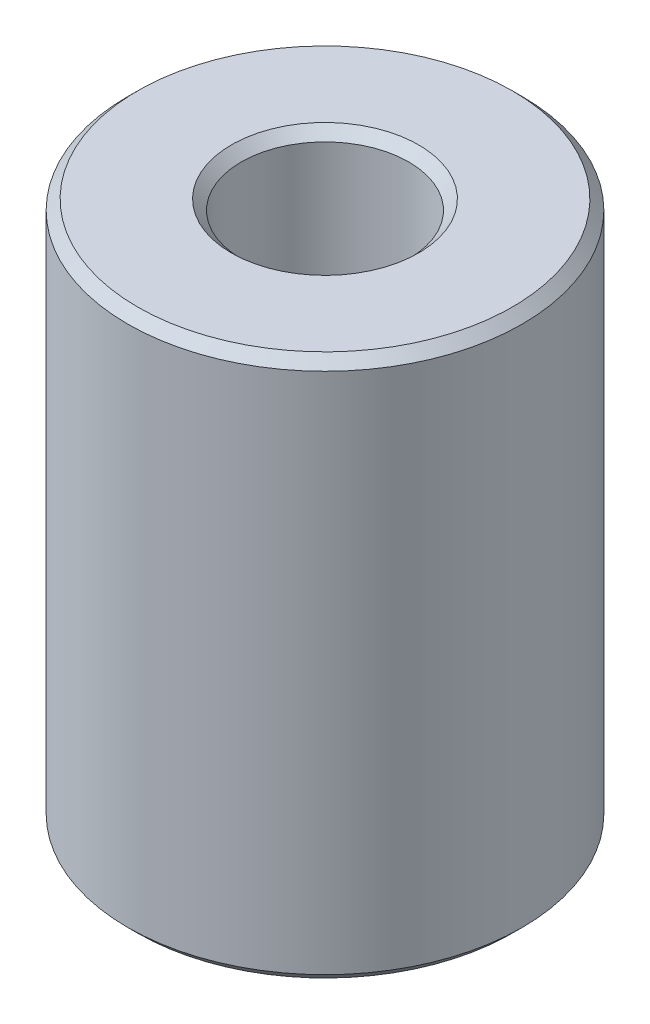
SolidWorks part; units mm, degrees
ref_plane "前视基准面" through (0, 0, 0) normal (0, 0, 1) x (1, 0, 0)
ref_plane "上视基准面" through (0, 0, 0) normal (0, 1, 0) x (1, 0, 0)
ref_plane "右视基准面" through (0, 0, 0) normal (1, 0, 0) x (0, 0, -1)
sketch "草图1" plane through (0, 0, 0) normal (0, 1, 0) x (1, 0, 0)
  circle A0 centre (0, 0) radius 20
  dimension "D1" = 40
extrude "凸台-拉伸1" add sketch "草图1" along normal blind 55
sketch "草图2" plane through (0, 55, 0) normal (0, 1, 0) x (1, 0, 0)
  circle A0 centre (0, 0) radius 8.5
  dimension "D1" = 17
extrude "切除-拉伸1" cut sketch "草图2" against normal blind 20
sketch "草图3" plane through (0, 0, 0) normal (0, -1, 0) x (1, 0, 0)
  circle A0 centre (0, 0) radius 10
  dimension "D1" = 20
extrude "切除-拉伸2" cut sketch "草图3" against normal blind 20
chamfer "倒角1" distance 1 angle 45 4 edges at (0, 55, 8.5) (0, 0, -10) (0, 55, 20) (0, 0, 20)
